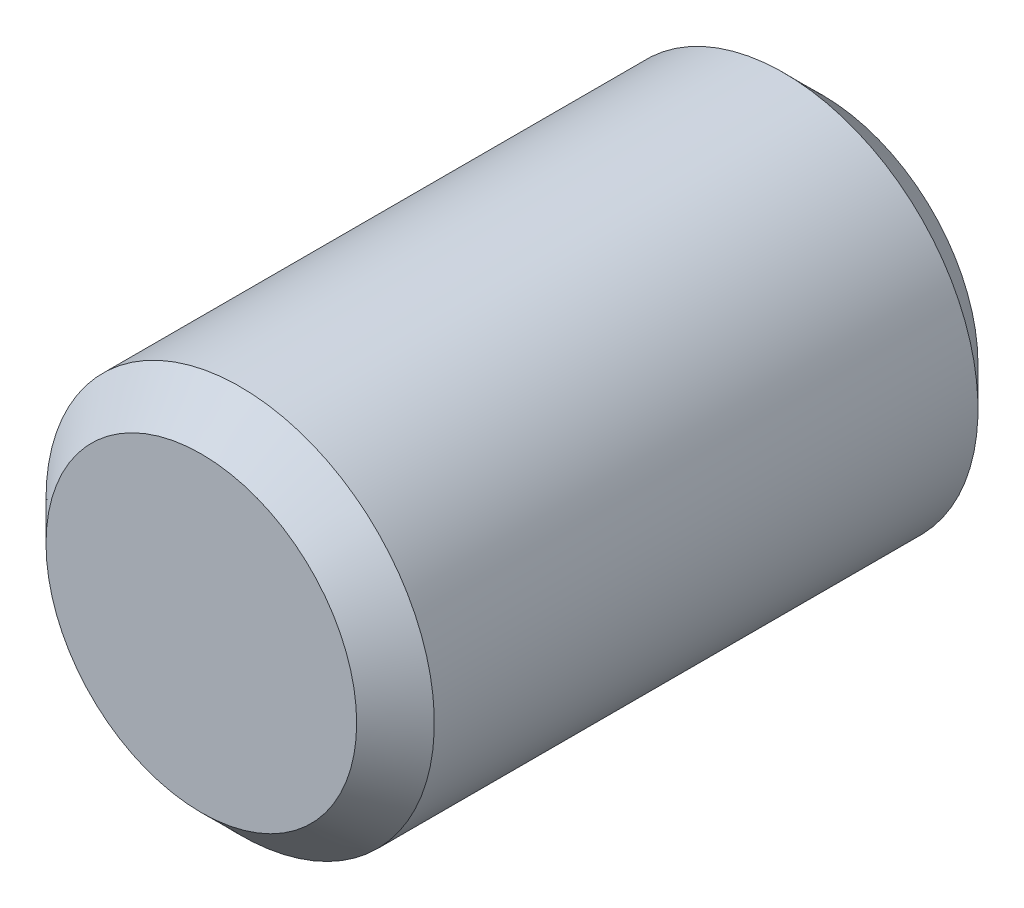
from build123d import *


with BuildPart() as part:
    # Sketch1 → Revolve1 (revolve)
    with BuildSketch(Plane.XZ, mode=Mode.PRIVATE) as revolve1_sk:
        Polygon((2, 8), (0, 8), (0, 0), (2, 0), (2.5, 0.5), (2.5, 7.5), align=None)
    revolve(revolve1_sk.sketch.rotate(Axis((0, 0, 8), (0, 0, -1)), 180), axis=Axis((0, 0, 8), (0, 0, -1)))


solid = part.part
